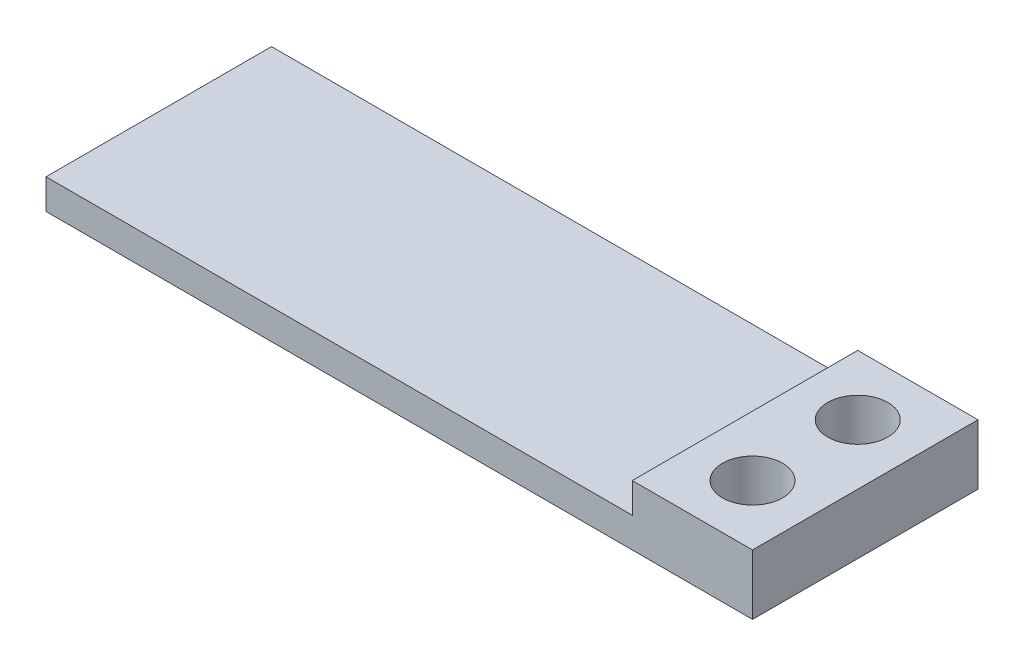
from build123d import *

# Parameters (mm, degrees)
EXTRUDE_1_DEPTH     = 7.5
CUT_EXTRUDE_1_REACH = 49.762
SKETCH_2_R          = 2


with BuildPart() as part:
    # 草图1 → 凸台-拉伸1 (new, symmetric)
    with BuildSketch(Plane.XY):
        Polygon((0, 0), (47, 0), (47, 4), (39, 4), (39, 2), (0, 2), align=None)
    extrude(amount=EXTRUDE_1_DEPTH, both=True)

    # 草图2 → 切除-拉伸1 (cut, up to next)
    with BuildSketch(Plane(origin=(0, 4, 0), x_dir=(1, 0, 0), z_dir=(0, 1, 0)), mode=Mode.PRIVATE) as cut_extrude_1_sk1:
        with Locations(Location((43, 3.5, 0), (0, 0, 180))):
            Circle(SKETCH_2_R)
    cut_extrude_1_tool1 = extrude(cut_extrude_1_sk1.sketch, amount=-CUT_EXTRUDE_1_REACH, mode=Mode.PRIVATE) & part.part
    # 草图2 → 切除-拉伸1 (cut, up to next)
    with BuildSketch(Plane(origin=(0, 4, 0), x_dir=(1, 0, 0), z_dir=(0, 1, 0)), mode=Mode.PRIVATE) as cut_extrude_1_sk2:
        with Locations(Location((43, -3.5, 0), (0, 0, 180))):
            Circle(SKETCH_2_R)
    cut_extrude_1_tool2 = extrude(cut_extrude_1_sk2.sketch, amount=-CUT_EXTRUDE_1_REACH, mode=Mode.PRIVATE) & part.part
    add(cut_extrude_1_tool1.solids().sort_by_distance((43, 4, -3.5))[0], mode=Mode.SUBTRACT)
    add(cut_extrude_1_tool2.solids().sort_by_distance((43, 4, 3.5))[0], mode=Mode.SUBTRACT)


solid = part.part
